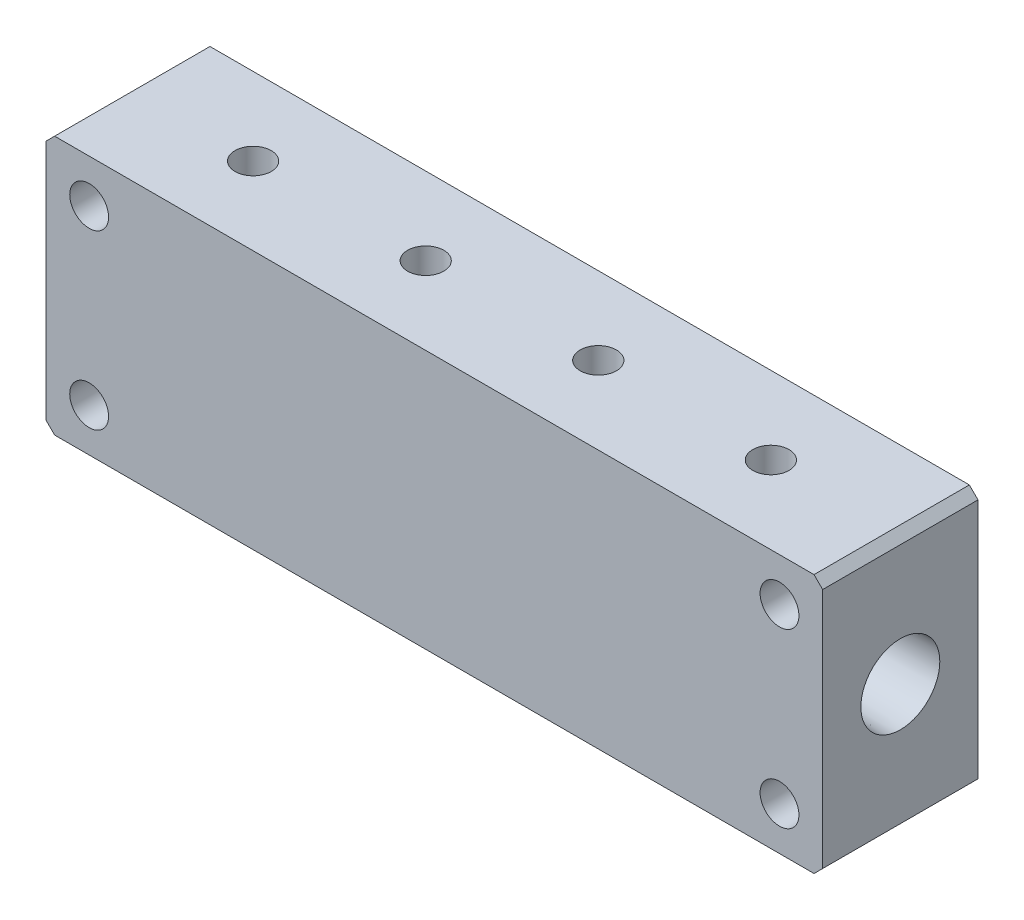
SolidWorks part; units mm, degrees
material "A6061"
ref_plane "前基準面" through (0, 0, 0) normal (0, 0, 1) x (1, 0, 0)
ref_plane "上基準面" through (0, 0, 0) normal (0, 1, 0) x (1, 0, 0)
ref_plane "右基準面" through (0, 0, 0) normal (1, 0, 0) x (0, 0, -1)
sketch "草图1" plane through (0, 0, 0) normal (0, 1, 0) x (1, 0, 0)
  line L1 (-45, -9) -> (45, -9)
  line L2 (-45, -9) -> (-45, 9)
  line L3 (-45, 9) -> (45, 9)
  line L4 (45, -9) -> (45, 9)
  line L5 (-45, -9) -> (45, 9) construction
  line L6 (-45, 9) -> (45, -9) construction
  point P0 (0, 0)
  dimension "D1" = 90
  dimension "D2" = 18
extrude "凸台-拉伸1" add sketch "草图1" along normal mid plane 30
hole_wizard "1/8 Rc 螺纹孔2" positions "草图2" profile "草图4" size "1/8" standard "GB"
sketch "草图2" plane through (45, 0, 0) normal (1, 0, 0) x (0, 0, -1)
  point P0 (0, 0)
sketch "草图4" plane through (45, 0, 0) normal (0, 1, 0) x (0, 0, -1)
  line L0 (0, 0) -> (0, 82.3734)
  line L1 (3.95, 80) -> (0, 82.3734)
  line L2 (-3.95, 80) -> (0, 82.3734) construction
  line L3 (3.95, 80) -> (3.95, 7.4)
  line L4 (3.95, 7.4) -> (4.3425, 7.4)
  line L5 (4.3425, 7.4) -> (4.5735, 0)
  line L6 (-4.3425, 7.4) -> (-4.5735, 0) construction
  line L7 (4.5735, 0) -> (0, 0)
  line L8 (0, -6.35) -> (0, 107.95) construction
  line L11 (-3.95, 7.4) -> (-4.3425, 7.4) construction
  dimension "螺纹孔钻头直径" = 7.9
  dimension "螺纹孔钻头深度" = 80
  dimension "螺纹直径" = 9.147
  dimension "螺纹角度" = 3.576
  dimension "螺纹深度" = 7.4
  dimension "导头角度" = 118
cosmetic thread "孔螺蚊线7"
hole_wizard "M5 螺纹孔1" positions "草图7" profile "草图8" tap size "M5" standard "GB" end condition through all
sketch "草图7" plane through (0, 15, 0) normal (0, 1, 0) x (1, 0, 0)
  line L0 (0, 0) -> (0, 19.2628) construction
  point P0 (30, 0)
  point P5 (10, 0)
  point P6 (-10, 0)
  point P7 (-30, 0)
  dimension "D2" = 20
  dimension "D1" = 4
cosmetic thread "孔螺蚊线3"
cosmetic thread "孔螺蚊线4"
cosmetic thread "孔螺蚊线5"
cosmetic thread "孔螺蚊线6"
sketch "草图8" plane through (30, 15, 0) normal (1, 0, 0) x (0, 0, 1)
  line L0 (0, 0) -> (0, 30)
  line L1 (0, 30) -> (2.1, 30)
  line L2 (2.1, 30) -> (2.1, 0)
  line L5 (2.1, 0) -> (0, 0)
  line L11 (0, -6.35) -> (0, 107.95) construction
  dimension "通孔螺纹孔钻头直径" = 4.2
  dimension "通孔螺纹孔钻头深度" = 30
hole_wizard "打孔尺寸(%根据)内六角圆柱头螺钉的类型1" positions "草图9" profile "草图10" counterbore size "M4" standard "GB" end condition through all
sketch "草图9" plane through (0, 0, -9) normal (0, 0, 1) x (1, 0, 0)
  line L0 (0, 25.1955) -> (0, 0) construction
  line L1 (0, 0) -> (-67.1651, 0) construction
  line L3 (45, 15) -> (-45, 15) construction
  point P0 (-40, 10)
  point P10 (-40, -10)
  point P11 (40, -10)
  point P12 (40, 10)
  dimension "D1" = 80
  dimension "D2" = 5
sketch "草图10" plane through (-40, 10, -9) normal (1, 0, 0) x (0, 1, 0)
  line L0 (0, 0) -> (0, 18)
  line L1 (0, 18) -> (2.25, 18)
  line L3 (2.25, 18) -> (2.25, 4.6)
  line L4 (2.25, 4.6) -> (4, 4.6)
  line L5 (4, 4.6) -> (4, 0)
  line L7 (4, 0) -> (0, 0)
  line L11 (0, -6.35) -> (0, 107.95) construction
  dimension "通孔孔直径" = 4.5
  dimension "通孔孔深度" = 18
  dimension "柱形沉头孔直径" = 8
  dimension "柱形沉头孔深度" = 4.6
chamfer "倒角1" distance 1 angle 45 4 edges at (45, -15, 0) (-45, -15, 0) (-45, 15, 0) (45, 15, 0)
